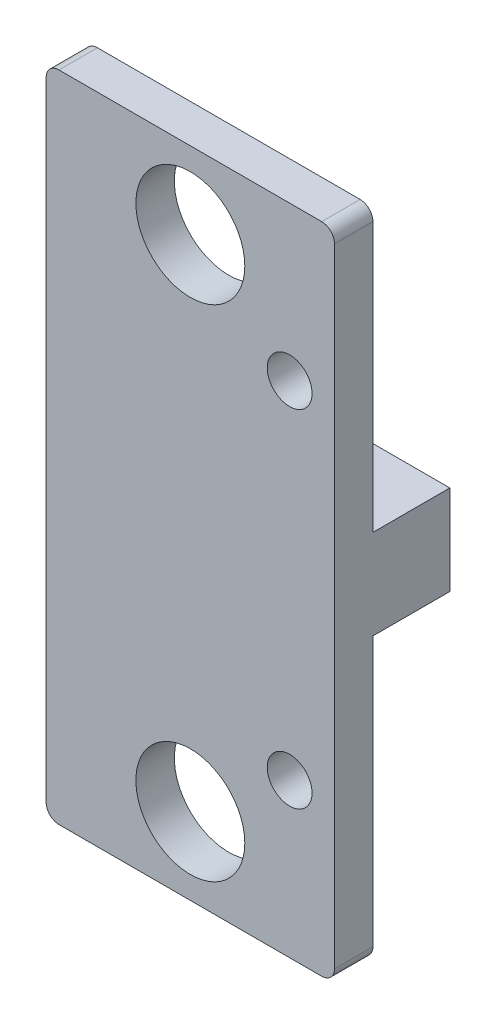
SolidWorks part; units mm, degrees
ref_plane "前视基准面" through (0, 0, 0) normal (0, 0, 1) x (1, 0, 0)
ref_plane "上视基准面" through (0, 0, 0) normal (0, 1, 0) x (1, 0, 0)
ref_plane "右视基准面" through (0, 0, 0) normal (1, 0, 0) x (0, 0, -1)
sketch "草图1" plane through (0, 0, 0) normal (0, 0, 1) x (1, 0, 0)
  line L1 (22.5, -46) -> (-22.5, -46)
  line L2 (22.5, -46) -> (22.5, 12)
  line L3 (22.5, 12) -> (-22.5, 12)
  line L4 (-22.5, -46) -> (-22.5, 12)
  line L5 (22.5, -46) -> (-22.5, 12) construction
  line L6 (22.5, 12) -> (-22.5, -46) construction
  circle A0 centre (0, 0) radius 8.5
  point P3 (0, -17)
  dimension "D1" = 17
  dimension "D2" = 12
  dimension "D3" = 45
  dimension "D4" = 46
extrude "凸台-拉伸1" add sketch "草图1" along normal blind 6
sketch "草图2" plane through (0, 0, 0) normal (0, 0, -1) x (-1, 0, 0)
  line L0 (22.5, 12) -> (22.5, -46) construction
  line L1 (-22.5, -46) -> (22.5, -46)
  line L2 (-22.5, -46) -> (-22.5, -32)
  line L3 (-22.5, -32) -> (22.5, -32)
  line L4 (22.5, -46) -> (22.5, -32)
  dimension "D1" = 14
extrude "凸台-拉伸2" add sketch "草图2" along normal blind 12
hole_wizard "M8x1.0 螺纹孔1" positions "3D草图1" profile "草图3" tap size "M8x1.0" standard "GB" end condition through all
sketch3d "3D草图1"
  line L0 (22.5, 12, 6) -> (-22.5, 12, 6) construction
  line L2 (22.5, -46, 6) -> (22.5, 12, 6) construction
  point P0 (15.5, -12, 6)
  dimension "D1" = 24
  dimension "D2" = 7
sketch "草图3" plane through (15.5, -12, 6) normal (1, 0, 0) x (0, -1, 0)
  line L0 (0, 0) -> (0, 18)
  line L1 (0, 18) -> (3.5, 18)
  line L2 (3.5, 18) -> (3.5, 0)
  line L5 (3.5, 0) -> (0, 0)
  line L11 (0, -6.35) -> (0, 107.95) construction
  dimension "通孔螺纹孔钻头直径" = 7
  dimension "通孔螺纹孔钻头深度" = 18
cosmetic thread "孔螺蚊线1" parameters "D2"=8
ref_plane "基准面1" through (0, -39, 0) normal (0, -1, 0) x (-1, 0, 0)
mirror "镜向1" about plane through (0, -39, 0) normal (0, -1, 0) of "凸台-拉伸1", "M8x1.0 螺纹孔1"
fillet "圆角1" radius 2 4 edges at (-22.5, 12, 3) (22.5, 12, 3) (22.5, -90, 3) (-22.5, -90, 3)
